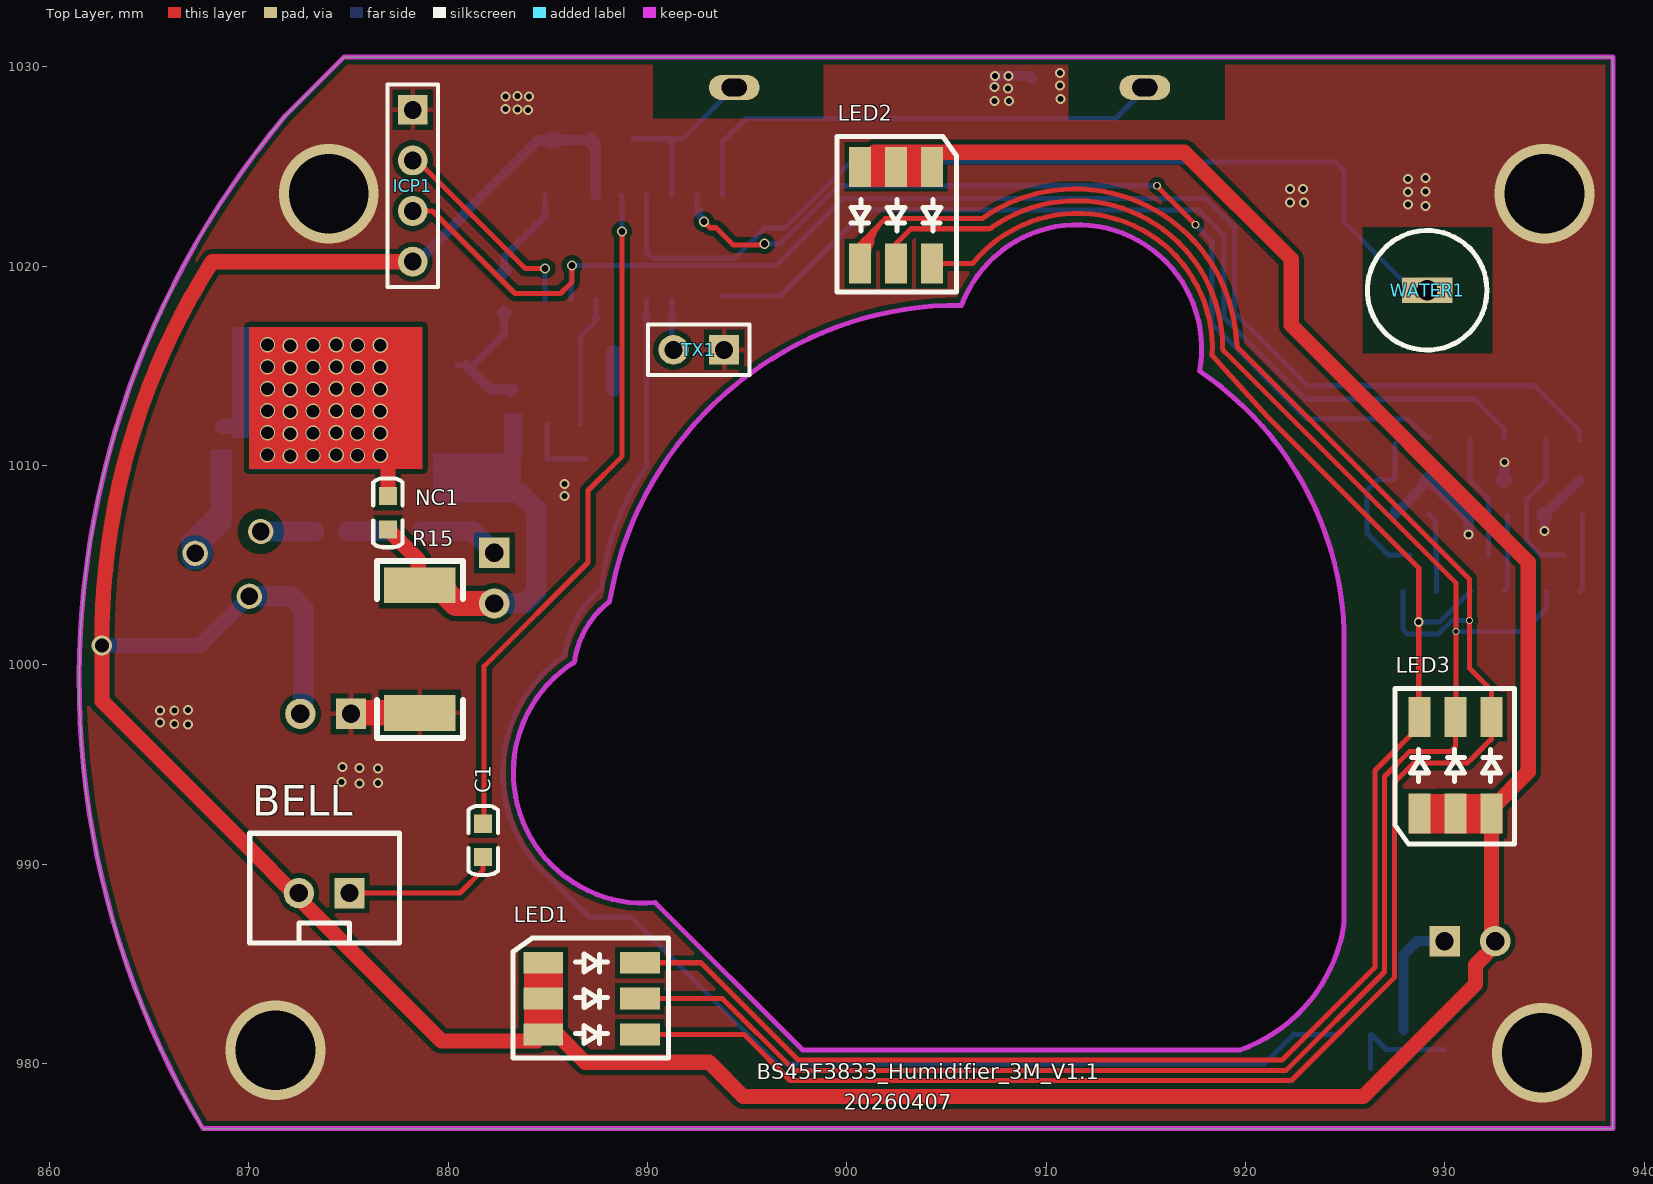
[diagram p0: Top Layer view]
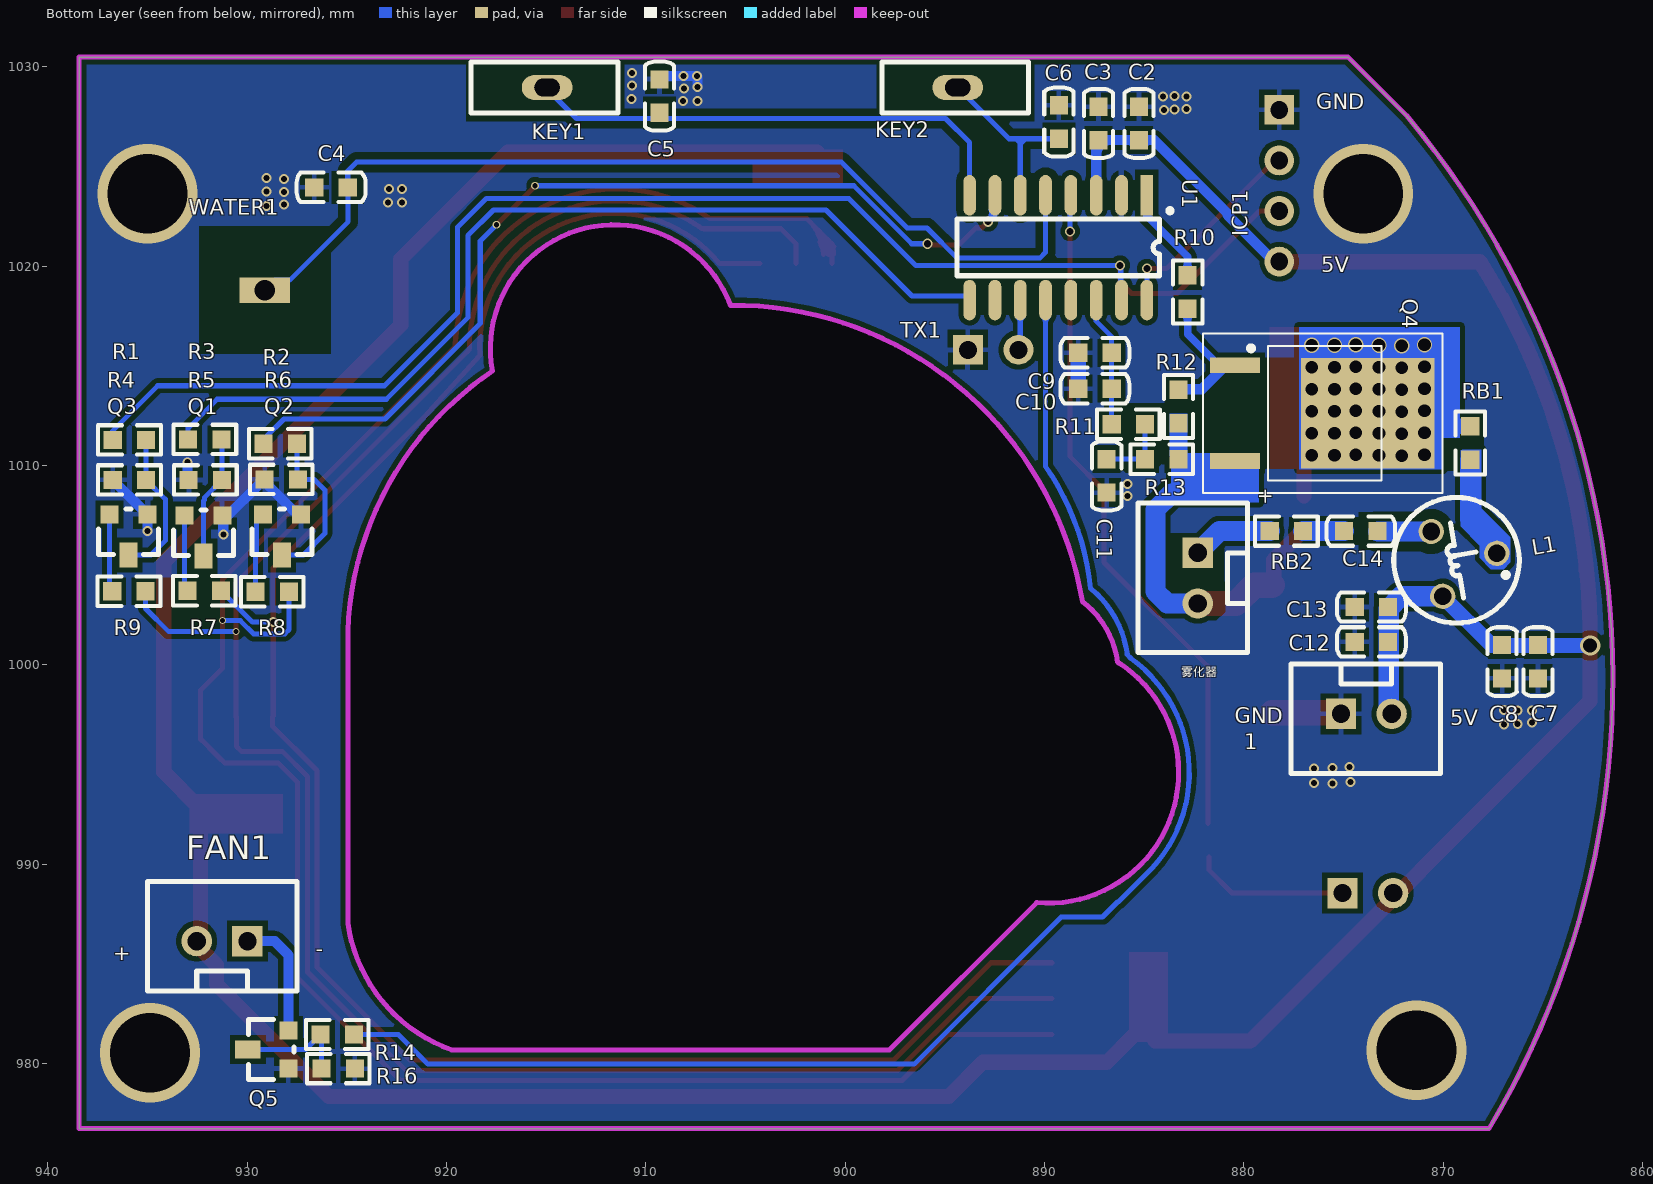
[diagram p1: Bottom Layer view, seen from below]
# Altium PCB MISC75988.PcbDoc
Units mm, origin at the board's own origin, x right, y up, seen from the top; angles counter-clockwise.
Board outline 76.94 x 53.76 mm, 2 copper layers (Top Layer, Bottom Layer); 52 components, 34 nets, 135 pads, 93 vias.

## Layer stack, top to bottom (the 12.6 mil dielectric is the usual default, probably not edited)
Top Solder: solder mask 0.0102, Solder Resist, Dk 3.5
Top Layer: signal copper 0.0356
Dielectric1: dielectric 0.32, FR-4, Dk 4.8
Bottom Layer: signal copper 0.0356
Bottom Solder: solder mask 0.0102, Solder Resist, Dk 3.5

## Board outline
867.709,976.722 cw(c905.383,999.236) 871.855,1027.557 874.776,1030.478 938.435,1030.478 938.435,976.725
cut-out: 897.779,980.678 890.397,988.06 cw(c889.83,994.586) 886.333,1000.125 cw(c890.932,999.485) 888.111,1003.173 cw(c905.647,1000.255) 905.764,1018.032 cw(c911.587,1015.853) 917.702,1014.73 cw(c908.483,1001.064) 924.957,1001.649 924.957,987.028 cw(c917.076,988.18) 919.75,980.678

## Design rules (kind name [scope] priority, off if disabled: settings)
Clearance Clearance_10 [InNet('NetB2_1')] p1: gap=0.635 ignorepadtopadclearanceinfootprint=FALSE except(0: Arc-Hole Track-Hole SMDPad-Hole THPad-Hole Via-Hole Fill-Hole Poly-Hole Region-Hole Text-Hole)
Clearance Clearance_9 [InNet('NetC14_2')] p2: gap=0.508 ignorepadtopadclearanceinfootprint=FALSE except(0: Arc-Hole Track-Hole SMDPad-Hole THPad-Hole Via-Hole Fill-Hole Poly-Hole Region-Hole Text-Hole)
Clearance Clearance_8 [InNet('K1')] p3: gap=0.381 ignorepadtopadclearanceinfootprint=FALSE except(0: Arc-Hole Track-Hole SMDPad-Hole THPad-Hole Via-Hole Fill-Hole Poly-Hole Region-Hole Text-Hole)
Clearance Clearance_7 [InNet('K2')] p4: gap=0.381 ignorepadtopadclearanceinfootprint=FALSE except(0: Arc-Hole Track-Hole SMDPad-Hole THPad-Hole Via-Hole Fill-Hole Poly-Hole Region-Hole Text-Hole)
Clearance Clearance_6 [InNet('WATER')] p5: gap=0.381 ignorepadtopadclearanceinfootprint=FALSE except(0: Arc-Hole Track-Hole SMDPad-Hole THPad-Hole Via-Hole Fill-Hole Poly-Hole Region-Hole Text-Hole)
Clearance Clearance_5 [InNet('NetB2_1')] p6: gap=0.508 ignorepadtopadclearanceinfootprint=FALSE except(0: Arc-Hole Track-Hole SMDPad-Hole THPad-Hole Via-Hole Fill-Hole Poly-Hole Region-Hole Text-Hole)
Clearance Clearance_4 [InNet('NetB2_2')] p7: gap=0.508 ignorepadtopadclearanceinfootprint=FALSE except(0: Arc-Hole Track-Hole SMDPad-Hole THPad-Hole Via-Hole Fill-Hole Poly-Hole Region-Hole Text-Hole)
Clearance Clearance_3 [InNet('NetB1_2')] p8: gap=0.508 ignorepadtopadclearanceinfootprint=FALSE except(0: Arc-Hole Track-Hole SMDPad-Hole THPad-Hole Via-Hole Fill-Hole Poly-Hole Region-Hole Text-Hole)
Clearance Clearance_2 [InNet('NetB1_1')] p9: gap=0.508 ignorepadtopadclearanceinfootprint=FALSE except(0: Arc-Hole Track-Hole SMDPad-Hole THPad-Hole Via-Hole Fill-Hole Poly-Hole Region-Hole Text-Hole)
Clearance Clearance_1 [InNet('+5V')] p10: gap=0.254 ignorepadtopadclearanceinfootprint=FALSE except(0: Arc-Hole Track-Hole SMDPad-Hole THPad-Hole Via-Hole Fill-Hole Poly-Hole Region-Hole Text-Hole)
Clearance [All] p11: gap=0.254 ignorepadtopadclearanceinfootprint=FALSE except(0: Arc-Hole Track-Hole SMDPad-Hole THPad-Hole Via-Hole Fill-Hole Poly-Hole Region-Hole Text-Hole)
ComponentClearance [All] p1 off: gap=0.254 collisioncheckmode=3 verticalgap=0.254 showdistances=FALSE
Height [All] p1 off: minheight=0 maxheight=25.4 prefheight=12.7
HoleSize [All] p1: absolutevalues=TRUE maxlimit=100 minlimit=0.025 maxpercent=80.000 minpercent=20.000
HoleToHoleClearance [All] p1: gap=0.152 allowstackedmicrovias=TRUE
MinimumSolderMaskSliver [All] p1: minsoldermaskwidth=0.102
PolygonConnect [All] p1: thpad.connectstyle=Relief thpad.reliefconductorwidth=0.254 thpad.reliefentries=4 thpad.polygonreliefangle="90 Angle" thpad.airgapwidth=0.254 smdpad.connectstyle=Relief smdpad.reliefconductorwidth=0.254 smdpad.reliefentries=4 smdpad.polygonreliefangle="90 Angle" smdpad.airgapwidth=0.254 via.connectstyle=Direct via.reliefconductorwidth=0.254 via.reliefentries=4 via.polygonreliefangle="90 Angle" via.airgapwidth=0.254
RoutingVias [All] p1: holewidth=0.711 width=1.27 viastyle="Through Hole" minholewidth=0.711 minwidth=1.27 maxholewidth=0.711 maxwidth=1.27
SilkToSilkClearance [All] p1: silktosilkclearance=0.051
SilkToSolderMaskClearance SilkscreenOverComponentPads [IsPad] p1: minsilkscreentomaskgap=0.051 clearancetoexposedcopper=TRUE
SolderMaskExpansion [All] p1: expansion=0.102 istentingtop=FALSE
Width GND [InNet('GND')] p1: maxlimit=1.524 minlimit=0.508 preferedwidth=0.508
Width +5V [InNet('+5V')] p2: maxlimit=1.524 minlimit=0.508 preferedwidth=0.762
Width Width_1 [All] p3: maxlimit=1.27 minlimit=0.254 preferedwidth=0.254
23 further rules are at their usual default settings.

## Components (designator, comment, footprint, x,y, rotation, side; value= is the part's Value field where it differs from the comment)
1 "POWER_5V" con2-wafer 875.132,997.534 r180 bottom
BELL "BELL" con2-wafer 875.055,988.543 r180 top
C1 "0.1uF" 0603C 881.761,990.346 r90 top value=104
C2 "0.1uF" 0603C 885.266,1026.312 r90 bottom value=106
C3 "0.1uF" 0603C 887.298,1026.312 r90 bottom value=104
C4 "CAP" 0603C 926.636,1023.944 r180 bottom value=8pf
C5 "CAP" 0603C 909.32,1029.36 r270 bottom value=8Pf
C6 "CAP" 0603C 889.283,1028.059 r270 bottom value=8Pf
C7 "CAP" 0603C 865.251,999.312 r90 bottom value=104
C8 "CAP" 0603C 867.054,999.312 r90 bottom value=10uF
C9 "22pF" 0603C 888.314,1015.644 r180 bottom
C10 "CAP" 0603C 888.314,1013.841 r180 bottom value=104
C11 "CAP" 0603C 886.892,1008.634 r90 bottom value=104
C12 "CAP" 0603C 874.446,1001.141 r180 bottom value=104
C13 "CAP" 0603C 874.446,1002.894 r180 bottom value=10uF
C14 "CAP" 0603C 874.979,1006.704 r180 bottom value="68nF 100V 5%"
FAN1 "FAN" con2-wafer 929.996,986.13 r0 bottom
ICP1 "ICP" HDR1X4 878.23,1027.836 r270 top
KEY1 "KEY1" TP2 903.529,1028.954 r0 bottom
KEY2 "KEY2" TP2 882.929,1028.954 r0 bottom
L1 "INDUCTOR" TREE 869.34,1005.357 r80 bottom
LED1 "RGB" LED-5050 884.784,985.037 r0 top
LED2 "RGB" LED-5050 904.265,1024.966 r270 top
LED3 "RGB" LED-5050 928.751,992.53 r90 top
NC1 "CAP" 0603C 876.986,1006.78 r90 top value=820pF
Q1 "S8050" SOT_23 931.24,1007.491 r0 bottom
Q2 "S8050" SOT_23 927.303,1007.542 r0 bottom
Q3 "S8050" SOT_23 934.999,1007.542 r0 bottom
Q4 "NCE0110K" TO252-3 876.046,1012.622 r180 bottom
Q5 "S8050" SOT_23 927.935,979.736 r90 bottom
R1 "2.2K" 0603R 936.752,1011.276 r180 bottom value=470R
R2 "2.2K" 0603R 929.186,1011.087 r180 bottom value=470R
R3 "15R" 0603R 932.967,1011.301 r180 bottom value=470R
R4 "2.2K" 0603R 936.752,1009.269 r180 bottom value=10K
R5 "2.2K" 0603R 932.942,1009.269 r180 bottom value=10K
R6 "2.2K" 0603R 929.132,1009.294 r180 bottom value=10K
R7 "100R/1206" 0603R 931.316,1003.706 r0 bottom value=150R
R8 "100R/1206" 0603R 927.909,1003.661 r0 bottom value=120R
R9 "100R/1206" 0603R 936.777,1003.681 r180 bottom value=100R
R10 "RES" 0603R 882.828,1019.531 r270 bottom value="30R 1%"
R11 "RES" 0603R 886.638,1012.063 r180 bottom value=20k
R12 "RES" 0603R 883.285,1012.114 r90 bottom value=2K
R13 "RES" 0603R 884.961,1010.31 r180 bottom value=20k
R14 "" 0603R 924.647,981.447 r0 bottom value=470R
R15 "RES" 2512 878.586,997.585 r90 top value=0.22ohm/0.5W
R16 "2.2K" 0603R 924.599,979.74 r0 bottom value=10K
RB1 "RES" 0603R 868.655,1011.961 r270 bottom value=0R
RB2 "RES" 0603R 878.713,1006.704 r180 bottom value=0R
TX1 "TX" HDR1X2 893.851,1015.797 r180 top
U1 "BS45F3833_16PIN" "NSOP 16" 889.406,1020.978 r270 bottom
WATER1 "WATER" Touch-Pad 929.118,1018.78 r0 top
雾化器 "" con2-wafer 882.322,1005.612 r270 bottom

## Footprints (in the part's own frame and the unit in brackets; to place one, negate y for a bottom-side part, rotate by r counter-clockwise, add the part's x,y. Pads: shape width x height; smd on the part's side, far side on the other; paste and mask are expansions set on the pad)
0603C [mil]
  rect 36x36 smd: 1(0,0) 2(66,0)
  silkscreen extent -35,-29 101,29
0603R [mil]
  rect 36x36 smd: 1(0,0) 2(66,0)
  silkscreen extent -29,-29 95,29
2512 [mm]
  rect 1.8x3.6 smd: 1(0,0) 2(6.4,0)
  silkscreen extent -1.27,-2.16 7.62,2.16
con2-wafer [mil]
  rect 60x60 hole 36: 1(0,0)
  round 60 hole 36: 2(100,0)
  silkscreen extent -98,-118 197,98
HDR1X2 [mm] "Connector; Header; 2 Position"
  rect 1.5x1.5 hole 0.9: 1(0,0)
  round 1.5 hole 0.9: 2(2.54,0)
  silkscreen extent -1.27,-1.27 3.81,1.27
HDR1X4 [mm] "Connector; Header; 4 Position"
  rect 1.5x1.5 hole 0.9: 1(0,0)
  round 1.5 hole 0.9: 2(2.54,0) 3(5.08,0) 4(7.62,0)
  silkscreen extent -1.27,-1.27 8.89,1.27
LED-5050 [mm]
  rect 2x1.1 smd: 1(-0.004,0.009) 2(-0.004,-1.791) 3(-0.004,-3.591) 4(4.846,0.009) 5(4.846,-1.791) 6(4.846,-3.591)
  silkscreen extent -1.52,-4.76 6.28,1.24
"NSOP 16" [mil]
  rect 80x25 smd: 1(-101.17,178.46)
  oval 80x25 smd: 2(-101.17,128.46) 3(-101.17,78.46) 4(-101.17,28.46) 5(-101.17,-21.54) 6(-101.17,-71.54) 7(-101.17,-121.54) 8(-101.17,-171.54) 9(105.83,-171.54) 10(105.83,-121.54) 11(105.83,-71.54) 12(105.83,-21.54) 13(105.83,28.46) 14(105.83,78.46) 15(105.83,128.46) 16(105.83,178.46)
  silkscreen extent -75,-196 58,228
SOT_23 [mil]
  rect 36x36 smd: 1(0.22,0.14) 3(75.22,0.14)
  rect 36x50 smd: 2(37.72,80.14)
  silkscreen extent -21,-11 97,79
TO252-3 [mm] "D-PAK, 3-Pads, Body 5.7x6.7mm (max),"
  rect 2.5x0.8 smd: 1(-4.4,2.4) 3(-4.4,-2.4)
  rect 6.7x5.55 smd: 2(2.25,0)
  silkscreen extent -6,-4 6,4
Touch-Pad [mil]
  rect 100x50 hole 40: 1(0,0)
  silkscreen extent -118,-118 118,118
TP2 [mil]
  oval 100x50 hole 35 slot 50 at 0 deg: 1(450,0)
  silkscreen extent 310,-50 600,50
TREE [mil]
  round 50 hole 35: 1(-70,40) 2(-5,-80) 3(60,40)
  silkscreen extent -129,-123 119,125

## Part data
1 BELL FAN1 TX1: library part "Header 2", "Header, 2-Pin"
C1 C2 C3: library part Cap, "Capacitor"
C4 C5 C6 C7 C8 C9 C10 C11 C12 C13 C14 NC1: library part CAP_4
ICP1: library part "Header 4", "Header, 4-Pin"
KEY1 KEY2 WATER1: library part Touch-Pad
L1: library part INDUCTOR5
LED1 LED2 LED3: library part RGB-CREE(5)
Q1 Q2 Q3 Q5: library part 2N3904, "NPN General Purpose Amplifier"
Q4: library part MOSFET-N, "N-Channel MOSFET"
R1 R2 R3 R4 R5 R6 R7 R8 R9 R14 R16: library part Res3, "Resistor"
R10 R11 R12 R13 R15 RB1 RB2: library part RES_4
雾化器: library part CRYSTAL_1

## Via types
v1: diameter 0.5, hole 0.3, Top Layer to Bottom Layer, tented both sides, 43 vias
v2: diameter 0.762, hole 0.635, Top Layer to Bottom Layer, 36 vias
v3: diameter 0.508, hole 0.356, Top Layer to Bottom Layer, tented both sides, 4 vias
v4: diameter 5, hole 4, Top Layer to Bottom Layer, 4 vias
v5: diameter 0.356, hole 0.254, Top Layer to Bottom Layer, 2 vias
v6: diameter 0.381, hole 0.254, Top Layer to Bottom Layer, 2 vias
v7: diameter 0.5, hole 0.356, Top Layer to Bottom Layer, tented both sides, 1 vias
v8: diameter 1.016, hole 0.711, Top Layer to Bottom Layer, 1 vias

## Nets (pads, with @x,y where several pads share a name; then routed paths per layer and width w, separated by ;. In a path a pad name is that pad's centre, name@x,y a point inside that pad or via, vN(x,y) a via of type N, cw(c..) or ccw(c..) an arc to the next point about the centre after c; other vN are vias at no path point)
+5V: 1.2 BELL.2 C2.1 C3.1 C7.2 C8.2 C12.2 C13.2 FAN1.2 ICP1.4 L1.1 LED1.1 LED1.2 LED1.3 LED2.1 LED2.2 LED2.3 LED3.1 LED3.2 LED3.3 U1.3 | length 226.6
  Top Layer w0.762: 862.838,1004.748 862.838,1005.002 ; ICP1.4 868.172,1020.216 ccw(c897.85,1001.269) 862.838,1005.002 ; LED1.3 885.49,981.446 886.885,980.052 886.892,980.059 893.089,980.059 894.809,978.34 ; LED1.1 884.46,984.726 884.46,981.126 879.678,981.126 862.635,998.169 862.635,1000.957 862.641,1000.963 cw(c897.85,1001.269) 862.838,1005.002 ; 896.696,978.34 894.809,978.34 ; LED2.3 901.407,1025.703 916.94,1025.703 922.299,1020.343 922.299,1017.041 934.187,1005.154 934.187,994.613 932.342,992.769 LED3.3 ; LED3.1 LED3.3@932.342,992.527 ; LED3.2 LED3.2@930.885,992.527 ; FAN1.2 932.536,985.923 931.545,984.933 931.545,983.971 925.914,978.34 894.809,978.34 ; FAN1.2@932.561,986.13 932.342,986.348 LED3.3
  Bottom Layer w0.508: ICP1.4@878.23,1019.962 880.821,1022.553 880.821,1022.629 884.504,1026.312 C2.1 C3.1 887.413,1026.197 U1.3 ; 884.776,1026.312 ccw(c884.776,1026.803) 885.123,1026.456 cw(c884.776,1026.803) 884.776,1026.312 ; 884.776,1026.312 cw(c884.776,1025.822) 885.123,1026.169 ccw(c884.776,1025.822) 884.776,1026.312 ; 885.757,1026.312 ccw(c885.757,1025.822) 885.41,1026.169 cw(c885.757,1025.822) 885.757,1026.312 ; 885.757,1026.312 cw(c885.757,1026.803) 885.41,1026.456 ccw(c885.757,1026.803) 885.757,1026.312 ; 886.808,1026.312 ccw(c886.808,1026.803) 887.155,1026.456 cw(c886.808,1026.803) 886.808,1026.312 ; 886.808,1026.312 cw(c886.808,1025.822) C3.1@887.155,1026.169 ; 886.808,1026.312 cw(c886.808,1025.822) C3.1@887.155,1026.169 ; C3.1@887.155,1026.169 cw(c886.53,1025.544) 887.413,1025.544 ccw(c886.53,1025.544) C3.1@887.155,1026.169
  Bottom Layer w0.762: v8(862.635,1000.963) 867.565,1000.963 L1.1
  Bottom Layer w1.016: L1.1 872.131,1003.43 872.744,1002.817 872.744,997.687 1.2
AD: C9.2 C10.2 R11.1 U1.14 | length 7.5
  Bottom Layer w0.254: R11.1 C10.2 C9.2 886.638,1016.457 887.413,1017.233 ; U1.14 887.413,1017.233 ; 887.413,1017.233 ccw(c887.171,1017.233) 887.307,1017.434 cw(c887.171,1017.233) 887.413,1017.233 ; 887.413,1017.233 cw(c887.656,1017.233) 887.52,1017.434 ccw(c887.656,1017.233) 887.413,1017.233
FAN: R14.1 U1.12 | length 77.2
  Bottom Layer w0.254: U1.12 889.953,1009.954 ccw(c900.914,1002.428) 887.692,1003.827 ccw(c890.935,999.866) 885.855,1000.501 885.668,1000.314 ccw(c889.822,994.582) 884.61,989.792 886.312,988.09 886.343,988.09 887.096,987.338 889.166,987.338 896.547,979.957 920.937,979.957 922.427,981.447 R14.1 ; 889.953,1017.132 ccw(c889.494,1017.132) 889.819,1017.457 cw(c889.494,1017.132) 889.953,1017.132 ; 889.953,1017.132 cw(c890.413,1017.132) 890.088,1017.457 ccw(c890.413,1017.132) 889.953,1017.132
GND: 1.1 C2.2 C3.2 C4.1 C5.1 C6.1 C7.1 C8.1 C9.1 C10.1 C11.1 C12.1 C13.1 ICP1.1 Q1.1 Q2.1 Q3.1 Q5.1 R4.1 R5.1 R6.1 R15.1 R16.1 TX1.1 U1.2 | length 17.7
  Top Layer w0.762: 1.1 1.1@875.182,997.585
  Top Layer w1.27: 1.1@875.182,997.585 R15.1
  Bottom Layer w0.508: v1(907.415,1028.979) 907.415,1029.513 v1(907.44,1029.538) v1(908.126,1029.538) 909.142,1029.538 C5.1 ; Q2.1@927.505,1007.54 927.505,1007.734 927.512,1007.741 927.706,1007.741 928.929,1008.964 928.929,1009.091 R6.1@929.033,1009.091 ; R6.1@929.481,1008.983 930.977,1007.487 Q1.1 ; Q1.1@931.189,1007.325 931.204,1007.311 v1(931.204,1006.531) ; R5.1@932.99,1009.317 v1(932.99,1010.156) ; Q3.1@934.974,1007.507 935.013,1007.469 v1(935.013,1006.695) ; Q3.1@935.021,1007.554 935.208,1007.741 935.224,1007.741 R4.1
  Bottom Layer w0.762: C10.1 C9.1 ; R6.1 R6.1@929.214,1009.213 ; R5.1 R5.1@932.99,1009.317 ; Q3.1@934.974,1007.507 Q3.1 Q3.1@935.021,1007.554
  other v1: 875.563,994.029 876.478,994.054 874.649,994.105 876.478,994.791 875.563,994.816 874.7,994.867 866.953,997.001 866.267,997.026 865.556,997.102 865.556,997.712 866.267,997.712 866.953,997.737 885.85,1008.456 885.85,1009.066 929.03,1023.01 928.167,1023.087 922.249,1023.188 922.934,1023.188 928.167,1023.722 929.03,1023.747 922.249,1023.874 922.884,1023.874 928.167,1024.357 929.03,1024.407 884.022,1027.836 883.488,1027.862 882.879,1027.887 907.415,1028.268 908.152,1028.268 910.717,1028.37 882.879,1028.497 884.072,1028.497 883.488,1028.522 908.101,1028.903 910.692,1029.056 910.692,1029.691
  other v4: 934.879,980.535 871.347,980.662 874.014,1023.62 935.006,1023.62
ICPCK: ICP1.3 R1.1 U1.15 | length 72.3
  Top Layer w0.254: ICP1.3 879.221,1022.756 883.361,1018.616 885.647,1018.616 886.221,1019.19 886.221,1020.029 v3(886.22,1020.03)
  Bottom Layer w0.254: U1.15 886.182,1018.328 886.182,1019.992 v3(886.22,1020.03) 896.459,1020.03 899.82,1023.391 918.007,1023.391 919.455,1021.944 919.455,1017.651 923.112,1013.993 934.491,1013.993 936.752,1011.733 R1.1
ICPDA: ICP1.2 U1.16 | length 10.5
  Top Layer w0.254: ICP1.2 878.459,1025.296 883.887,1019.868 v3(884.874,1019.868)
  Bottom Layer w0.254: U1.16@884.874,1018.291 v3(884.874,1019.868)
K1: C6.2 KEY2.1 U1.6 | length 9.6
  Bottom Layer w0.254: C6.2 890.946,1026.382 ; U1.6 891.223,1026.105 ; KEY2.1@894.156,1029.157 894.156,1028.751 891.788,1026.382 891.44,1026.382 ; 890.946,1026.382 891.44,1026.382 ; 890.946,1026.382 891.223,1026.105 ; 891.223,1026.105 891.223,1026.166 891.44,1026.382
K2: C5.2 KEY1.1 U1.8 | length 25
  Bottom Layer w0.254: U1.8 893.763,1026.199 894.969,1027.405 910.158,1027.405 913.486,1027.405 KEY1.1@915.01,1028.929
L_B: LED1.6 LED2.6 LED3.6 R8.1 | length 124.6
  Top Layer w0.254: LED1.6 894.856,981.446 897.158,979.144 922.317,979.144 927.491,984.317 927.491,994.115 928.454,995.078 931.146,995.078 931.367,995.299 931.741,995.673 932.115,996.047 932.342,996.274 LED3.6 932.342,998.724 931.248,999.818 v5(931.248,1002.211) 931.248,1004.282 919.569,1015.962 ccw(c911.464,1015.757) 906.78,1022.375 901.929,1022.375 900.674,1021.121 ; LED2.6@900.59,1020.716 ccw(c899.688,1022.278) 901.43,1021.811 ; LED2.6@900.606,1020.725 ccw(c900.313,1021.386) 901.012,1021.199 ; LED2.6 900.674,1021.121 ; LED2.6@900.717,1020.496 ccw(c900.122,1021.527) 901.271,1021.219 ; 900.994,1021.134 ccw(c901.442,1021.013) LED2.6@901.04,1020.782 ; 900.674,1021.121 cw(c900.527,1021.121) 900.565,1020.979 ccw(c900.527,1021.121) 900.674,1021.121 ; 900.674,1021.121 ccw(c900.821,1021.121) 900.783,1020.979 cw(c900.821,1021.121) 900.674,1021.121 ; LED2.6@900.589,1020.57 cw(c901.714,1020.57) 900.918,1021.365 ccw(c901.714,1020.57) LED2.6@900.589,1020.57 ; LED2.6@900.843,1020.57 cw(c902.581,1020.57) 901.352,1021.799 ccw(c902.581,1020.57) LED2.6@900.843,1020.57 ; LED2.6@901.097,1020.57 cw(c903.448,1020.57) 901.786,1022.232 ccw(c903.448,1020.57) LED2.6@901.097,1020.57
  Bottom Layer w0.254: R8.1 927.909,1001.754 928.116,1001.547 929.691,1001.547 930.354,1002.211 v5(931.248,1002.211)
L_G: LED1.5 LED2.5 LED3.5 R9.2 | length 107.8
  Top Layer w0.254: LED1.5 893.774,983.246 897.368,979.652 922.048,979.652 926.983,984.586 926.983,994.395 928.243,995.655 930.3,995.655 930.542,995.897 LED3.5 ; LED2.5 902.474,1021.117 903.224,1021.867 907.105,1021.867 ccw(c907.104,1022.121) 907.251,1021.914 cw(c911.507,1015.92) 918.858,1015.909 ccw(c919.112,1015.91) 918.86,1015.879 918.871,1015.793 918.932,1015.731 ccw(c919.112,1015.91) 918.945,1015.719 930.556,1004.107 v5(930.556,1001.655) LED3.5@930.556,997.377
  Bottom Layer w0.254: v5(930.556,1001.655) 933.939,1001.655 935.101,1002.817 R9.2
L_R: LED1.4 LED2.4 LED3.4 R7.1 | length 98.9
  Top Layer w0.254: LED1.4 892.693,985.046 897.579,980.16 921.838,980.16 926.505,984.827 926.505,994.689 928.742,996.927 LED3.4 ; LED2.4 906.313,1020.12 cw(c911.581,1015.881) 918.333,1015.523 921.114,1012.431 921.121,1012.424 921.124,1012.42 928.696,1004.848 v1(928.696,1002.131) LED3.4@928.696,997.423
  Bottom Layer w0.254: v1(928.696,1002.131) 929.741,1002.131 R7.1
NetBELL_1: BELL.1 C1.1 | length 8
  Top Layer w0.254: BELL.1 880.596,988.543 ; 880.721,988.668 880.596,988.543 ; C1.1 881.761,989.708 880.596,988.543
NetC1_2: C1.2 U1.4 | length 34.4
  Top Layer w0.254: C1.2@881.812,992.022 881.812,999.922 887.019,1005.129 887.019,1008.736 888.721,1010.437 v7(888.721,1021.74)
  Bottom Layer w0.254: U1.4 888.721,1023.511 v7(888.721,1021.74)
NetC11_2: C11.2 R11.2 R13.1 | length 3.7
  Bottom Layer w0.254: R11.2 R13.1 C11.2
NetC14_1: C14.1 RB2.2 | length 2.1
  Bottom Layer w1.016: C14.1 RB2.2
NetC14_2: C14.2 L1.3 | length 2.7
  Bottom Layer w1.016: L1.3 C14.2@873.281,1006.682
NetFAN1_1: FAN1.1 Q5.3 | length 6.1
  Bottom Layer w0.508: Q5.3 927.938,985.444 928.624,986.13 FAN1.1
NetL1_2: L1.2 RB1.2 | length 5.3
  Bottom Layer w1: L1.2 867.317,1005.95 868.655,1007.288 RB1.2
NetNC1_1: NC1.1 Q4.3 R12.1 R13.2 R15.2 雾化器.2 | length 21
  Top Layer w0.762: NC1.1 878.51,1005.256 878.51,1004.061 R15.2
  Top Layer w1.27: R15.2 879.486,1003.985 880.399,1003.072 雾化器.2
  Bottom Layer w0.254: Q4.3@879.322,1009.985 cw(c879.482,1004.248) 879.779,1009.98 880.021,1010.222 Q4.3 ; R13.2@883.196,1010.222 R13.2
  Bottom Layer w0.762: Q4.3 R13.2@883.196,1010.222 ; 883.285,1008.634 R13.2
  Bottom Layer w1.016: 雾化器.2 883.844,1003.072 884.439,1003.667 884.439,1007.784 883.641,1008.583
NetNC1_2: NC1.2 Q4.2 RB1.1 | length 14.2
  Top Layer w0.762: v2(876.605,1010.501) 876.986,1010.12 NC1.2
  Bottom Layer w0.254: Q4.2@873.136,1011.961 Q4.2
  Bottom Layer w0.762: RB1.1 Q4.2@873.136,1011.961 ; Q4.2@870.779,1013.237 ccw(c870.131,1013.734) v2(870.941,1013.841) ; Q4.2@870.779,1013.237 ccw(c870.131,1013.734) v2(870.941,1013.841) ; Q4.2@870.779,1013.237 ccw(c870.131,1013.734) v2(870.941,1013.841) ; Q4.2@870.91,1013.364 ccw(c871.414,1013.074) v2(870.941,1012.736) ; Q4.2@870.91,1013.364 ccw(c871.414,1013.074) v2(870.941,1012.736) ; Q4.2@870.91,1013.364 ccw(c871.414,1013.074) v2(870.941,1012.736) ; v2(870.941,1012.736) ccw(c870.75,1013.862) Q4.2@871.681,1013.2 ; v2(870.941,1012.736) ccw(c870.75,1013.862) Q4.2@871.681,1013.2 ; v2(870.941,1012.736) ccw(c870.75,1013.862) Q4.2@871.681,1013.2
  other v2: 872.084,1010.476 870.941,1010.526 873.227,1010.501 874.395,1010.526 875.462,1010.501 872.084,1011.58 873.227,1011.606 875.462,1011.606 876.605,1011.606 870.941,1011.631 874.395,1011.631 872.084,1012.685 873.227,1012.711 875.462,1012.711 876.605,1012.711 874.395,1012.736 872.084,1013.79 873.227,1013.816 875.462,1013.816 876.605,1013.816 874.395,1013.841 872.084,1014.895 870.941,1014.946 873.227,1014.92 874.395,1014.946 875.462,1014.92 876.605,1014.92 872.084,1016 873.227,1016.025 875.462,1016.025 876.605,1016.025 870.941,1016.051 874.395,1016.051
NetQ1_2: Q1.2 R3.2 R5.2 | length 6.2
  Bottom Layer w0.254: R3.2 931.266,1011.276 R5.2 932.155,1008.38 932.155,1008.253 932.198,1008.209 Q1.2
NetQ1_3: Q1.3 R7.2 | length 3.8
  Bottom Layer w0.254: R7.2 933.151,1003.864 Q1.3
NetQ2_2: Q2.2 R2.2 R6.2 | length 8.2
  Bottom Layer w0.254: R2.2 927.51,1009.349 R6.2 926.643,1009.294 926.109,1008.761 926.109,1006.577 927.18,1005.506 Q2.2
NetQ2_3: Q2.3 R8.2 | length 4
  Bottom Layer w0.254: Q2.3 929.544,1007.208 929.544,1005.62 929.586,1005.579 R8.2
NetQ3_2: Q3.2 R1.2 R4.2 | length 7.6
  Bottom Layer w0.254: R1.2 R4.2 934.11,1008.304 934.11,1006.221 934.825,1005.506 Q3.2
NetQ3_3: Q3.3 R9.1 | length 3.9
  Bottom Layer w0.254: R9.1 936.91,1003.814 Q3.3
NetQ4_1: Q4.1 R10.2 R12.2 | length 10.6
  Bottom Layer w0.254: Q4.1@880.91,1015.022 Q4.1 Q4.1@881.265,1015.022
  Bottom Layer w0.381: Q4.1@881.265,1015.022 882.828,1016.584 R10.2 ; 882.828,1017.21 ccw(c882.184,1017.21) 882.639,1017.666 cw(c882.184,1017.21) 882.828,1017.21 ; 882.828,1017.21 cw(c883.472,1017.21) 883.016,1017.666 ccw(c883.472,1017.21) 882.828,1017.21
  Bottom Layer w0.508: Q4.1@880.91,1015.022 882.117,1013.816 R12.2@883.285,1013.816 ; 882.733,1013.816 cw(c882.733,1013.238) 883.141,1013.647 ccw(c882.733,1013.238) 882.733,1013.816
NetQ5_2: Q5.2 R14.2 R16.2 | length 5.7
  Bottom Layer w0.254: R16.2 926.275,981.4 R14.2 927.077,980.694 Q5.2
NetRB2_1: RB2.1 雾化器.1 | length 4.1
  Bottom Layer w1.016: RB2.1 881.23,1006.704 雾化器.1
PWM: R10.1 U1.1 | length 7.7
  Bottom Layer w0.254: U1.1 884.873,1022.516 ; 884.873,1022.516 ccw(c884.677,1022.516) 884.777,1022.685 cw(c884.677,1022.516) 884.873,1022.516 ; 884.873,1022.516 cw(c885.07,1022.516) 884.97,1022.685 ccw(c885.07,1022.516) 884.873,1022.516
  Bottom Layer w0.381: R10.1 882.828,1020.47 884.873,1022.516 ; 882.828,1020.174 ccw(c883.472,1020.174) 883.016,1019.719 cw(c883.472,1020.174) 882.828,1020.174 ; 882.828,1020.174 cw(c882.184,1020.174) 882.639,1019.719 ccw(c882.184,1020.174) 882.828,1020.174
RGB_B: R2.1 U1.7 | length 52.5
  Top Layer w0.254: v3(892.835,1022.223) 893.14,1021.918 893.445,1021.918 894.309,1021.055 v3@895.756,1021.055 ; v6@915.556,1024.014 v6(917.499,1022.071) ; 893.052,1022.006 cw(c893.269,1022.223) 892.962,1022.223 ccw(c893.269,1022.223) 893.052,1022.006 ; 893.052,1022.006 ccw(c892.835,1021.789) 892.835,1022.096 cw(c892.835,1021.789) 893.052,1022.006 ; v6@915.632,1024.026 ccw(c915.847,1024.026) 915.695,1023.875 cw(c915.847,1024.026) v6@915.632,1024.026
  Bottom Layer w0.254: U1.7@892.505,1023.548 U1.7 892.493,1022.565 v3(892.835,1022.223) ; U1.7@892.538,1022.895 cw(c892.205,1022.556) 892.68,1022.56 ; v3(895.872,1021.117) 896.668,1021.117 899.577,1024.026 v6@915.543,1024.026 ; v6(917.499,1022.071) 918.312,1021.257 918.312,1017.111 923.093,1012.33 928.154,1012.33 929.081,1011.403 R2.1@929.259,1011.403 ; 892.619,1022.44 cw(c892.402,1022.223) 892.708,1022.223 ccw(c892.402,1022.223) 892.619,1022.44 ; 892.619,1022.44 ccw(c892.835,1022.657) 892.835,1022.35 cw(c892.835,1022.657) 892.619,1022.44 ; 892.682,1022.489 cw(c892.417,1022.335) v3@892.713,1022.256 ; 892.682,1022.489 ccw(c892.948,1022.642) v3@892.868,1022.346 ; 892.682,1022.489 cw(c892.417,1022.335) v3@892.713,1022.256 ; 892.682,1022.489 ccw(c892.948,1022.642) v3@892.868,1022.346 ; 892.682,1022.489 cw(c892.417,1022.335) v3@892.713,1022.256 ; 892.682,1022.489 ccw(c892.948,1022.642) v3@892.868,1022.346 ; v3(892.835,1022.223) cw(c893.262,1022.65) 892.678,1022.802 ccw(c893.262,1022.65) v3(892.835,1022.223)
  other v6: 915.568,1024.026
RGB_R: R3.1 U1.9 | length 48.5
  Bottom Layer w0.254: U1.9@893.763,1018.5 896.656,1018.5 900.963,1022.807 917.651,1022.807 918.934,1021.524 918.934,1017.41 923.029,1013.315 931.512,1013.315 932.967,1011.86 R3.1
TX: TX1.2 U1.11 | length 4
  Bottom Layer w0.254: U1.11 891.223,1015.885 TX1.2 ; 891.223,1017.132 ccw(c890.764,1017.132) 891.089,1017.457 cw(c890.764,1017.132) 891.223,1017.132 ; 891.223,1017.132 cw(c891.683,1017.132) 891.358,1017.457 ccw(c891.683,1017.132) 891.223,1017.132
WATER: C4.2 U1.5 WATER1.1 | length 48.3
  Bottom Layer w0.254: U1.5 889.953,1020.685 890.245,1020.394 894.385,1020.394 895.901,1021.911 896.892,1021.911 900.188,1025.207 924.522,1025.207 924.96,1024.77 C4.2 924.94,1023.924 924.94,1022.224 927.876,1019.288 928.61,1019.288 WATER1.1
pads on no net: U1.10 U1.13

## Polygon pours and split planes (outlines as drawn)
GND on Top Layer "GND_L01_P000" (solid, remove dead copper, pour order 0): 870.653,1033.279 940.096,1033.279 941.214,1032.161 941.214,977.932 938.242,974.96 866.487,974.96 859.654,981.793 859.654,1013.518 860.848,1014.711 860.848,1023.728 870.653,1033.533
GND on Bottom Layer "GND_L02_P005" (solid, remove dead copper, pour order 5): 939.292,1033.678 868.02,1033.678 858.647,1024.306 858.647,980.211 863.956,974.903 939.47,974.903 944.27,979.703 944.27,1029.132 939.47,1033.932

## Keep-outs
Keep-Out Layer:
  lines w0.254: 867.709,976.722 cw(c905.383,999.236) 871.855,1027.557 874.776,1030.478 938.435,1030.478 938.435,976.725 ; 867.715,976.725 938.428,976.725 ; 919.75,980.678 ccw(c917.076,988.18) 924.957,987.028 ; 919.75,980.678 898.55,980.678 897.779,980.678 890.397,988.06 cw(c889.83,994.586) 886.333,1000.125 cw(c890.932,999.485) 888.111,1003.173 cw(c905.647,1000.255) 905.764,1018.032 cw(c911.587,1015.853) 917.702,1014.73 cw(c908.483,1001.064) 924.957,1001.649 924.957,987.028

## Other copper
Top Layer:
  rectangle net NetNC1_2: 870.026,1009.828 878.713,1016.94
  rectangle net +5V: 900.125,1023.976 904.646,1025.855
  rectangle net +5V: 883.818,981.177 885.774,985.596
  rectangle net +5V: 928.218,991.54 932.891,993.521
  pour cut-out: 925.881,1021.944 932.383,1021.944 932.383,1015.619 925.881,1015.619
  pour cut-out: 918.997,1030.389 918.997,1027.317 911.123,1027.317 911.123,1030.389
  pour cut-out: 898.855,1030.402 898.855,1027.379 890.27,1027.379 890.27,1030.402
Bottom Layer:
  rectangle net NetNC1_1: 882.828,1010.437 883.742,1012.596
  rectangle net NetNC1_2: 869.163,1011.377 877.24,1016.94
  rectangle net NetNC1_2: 870.026,1009.802 877.24,1016.66
  rectangle net NetNC1_1: 879.246,1008.126 883.59,1010.615
  region net NetL1_2: 869.086,1010.768 869.061,1010.793 868.096,1010.793 868.096,1007.847 866.648,1006.399 866.648,1005.129 866.978,1004.799 867.613,1004.799 868.172,1005.357 868.172,1005.967 869.137,1006.932 869.137,1010.768 869.061,1010.768 869.036,1010.793
  pour cut-out: 868.959,1011.479 868.731,1011.25 867.943,1011.25 867.943,1010.996 868.065,1011.118 869.378,1011.118 869.378,1009.84 869.264,1009.726 869.287,1009.703 869.787,1009.703 869.787,1011.099 869.767,1011.118
  pour cut-out: 881.38,1002.208 880.923,1002.665 880.923,1004.164 882.193,1004.164 882.447,1003.91 882.447,1002.208 881.355,1002.208
  pour cut-out: 931.487,1004.566 931.393,1004.472 931.393,1002.545 931.081,1002.233 933.104,1002.233 934.39,1003.519 934.39,1004.392 933.051,1004.392 932.993,1004.45
  pour cut-out: 881.758,1010.89 881.727,1010.92 881.727,1013.312 883.763,1013.312 883.996,1013.079 884.047,1013.13 886.249,1013.13 886.249,1010.191 886.384,1010.056 885.927,1009.599 884.25,1009.599 884.25,1009.929 883.234,1010.945 882.32,1010.945
  pour cut-out: 925.779,1015.568 932.434,1015.568 932.434,1022.02 925.779,1022.02
  pour cut-out: 919.048,1027.227 919.048,1030.402 911.073,1030.402 911.073,1027.227
  pour cut-out: 890.499,1027.227 890.499,1030.44 898.436,1030.44 898.449,1030.427 898.449,1027.227
  pour cut-out: 881.71,1014.679 880.974,1015.416 877.265,1015.416 877.265,1009.828 877.24,1009.802 878.738,1009.828 879.094,1009.929 880.923,1009.929 881.761,1010.615
  pour cut-out: 880.974,1005.817 881.092,1005.935 881.272,1005.935 881.965,1006.628 883.666,1006.628 883.666,1004.24 881.075,1004.24 880.999,1004.164 880.98,1004.164 880.974,1004.17

## Silkscreen, mask and mechanical layers (free items; w line width, h text height)
Top Overlay:
  text "BS45F3833_Humidifier_3M_V1.1" at 895.477,979.195 h0.76
  text "20260407" at 899.846,977.671 h0.76
Bottom Overlay:
  text "GND" at 876.376,1027.862 h0.76
  text "5V" at 876.122,1019.683 h0.76
  text "+" at 879.246,1007.999 h0.76 r90
  text "GND" at 880.466,997.052 h0.76
  text "5V" at 869.645,996.95 h0.76
  text "-" at 926.567,985.952 h0.76 r180
  text "+" at 935.852,985.165 h0.76
Top Solder:
  rectangle: 870.052,1009.853 877.316,1016.94
Bottom Solder:
  rectangle: 869.188,1011.352 877.265,1016.94